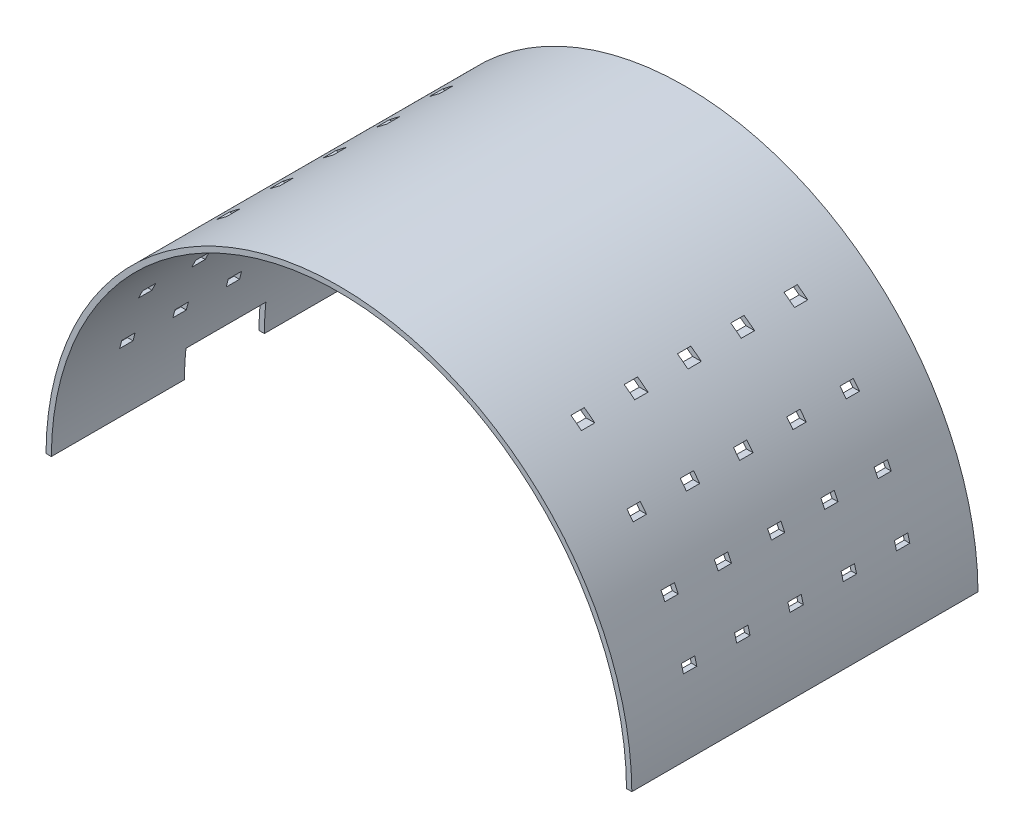
SolidWorks part; units mm, degrees
ref_plane "前视基准面" through (0, 0, 0) normal (0, 0, 1) x (1, 0, 0)
ref_plane "上视基准面" through (0, 0, 0) normal (0, 1, 0) x (1, 0, 0)
ref_plane "右视基准面" through (0, 0, 0) normal (1, 0, 0) x (0, 0, -1)
other "Configuration Table"
sketch "草图1" plane through (0, 0, 0) normal (0, 0, 1) x (1, 0, 0)
  line L0 (0.0023, 1) -> (4.0023, 1)
  line L1 (435.9977, 1) -> (439.9977, 1)
  arc A0 (439.9977, 1) -> (0.0023, 1) centre (220, 0) ccw
  arc A1 (4.0023, 1) -> (435.9977, 1) centre (220, 0) cw
  point P0 (0, 0)
  dimension "D1" = 220
  dimension "D2" = 216
  dimension "D3" = 4
extrude "凸台-拉伸1" add sketch "草图1" against normal mid plane 260
sketch "草图2" plane through (0, 0, 0) normal (1, 0, 0) x (0, 0, -1)
  line L0 (85, 52) -> (85, 58)
  line L1 (85, 58) -> (75, 58)
  line L2 (75, 58) -> (75, 52)
  line L3 (75, 52) -> (85, 52)
  line L4 (45, 52) -> (45, 58)
  line L5 (45, 58) -> (35, 58)
  line L6 (35, 58) -> (35, 52)
  line L7 (35, 52) -> (45, 52)
  line L8 (5, 52) -> (5, 58)
  line L9 (5, 58) -> (-5, 58)
  line L10 (-5, 58) -> (-5, 52)
  line L11 (-5, 52) -> (5, 52)
  line L12 (-35, 52) -> (-35, 58)
  line L13 (-35, 58) -> (-45, 58)
  line L14 (-45, 58) -> (-45, 52)
  line L15 (-45, 52) -> (-35, 52)
  line L16 (-75, 52) -> (-75, 58)
  line L17 (-75, 58) -> (-85, 58)
  line L18 (-85, 58) -> (-85, 52)
  line L19 (-85, 52) -> (-75, 52)
  line L20 (85, 92) -> (85, 98)
  line L21 (85, 98) -> (75, 98)
  line L22 (75, 98) -> (75, 92)
  line L23 (75, 92) -> (85, 92)
  line L24 (45, 92) -> (45, 98)
  line L25 (45, 98) -> (35, 98)
  line L26 (35, 98) -> (35, 92)
  line L27 (35, 92) -> (45, 92)
  line L28 (5, 92) -> (5, 98)
  line L29 (5, 98) -> (-5, 98)
  line L30 (-5, 98) -> (-5, 92)
  line L31 (-5, 92) -> (5, 92)
  line L32 (-35, 92) -> (-35, 98)
  line L33 (-35, 98) -> (-45, 98)
  line L34 (-45, 98) -> (-45, 92)
  line L35 (-45, 92) -> (-35, 92)
  line L36 (-75, 92) -> (-75, 98)
  line L37 (-75, 98) -> (-85, 98)
  line L38 (-85, 98) -> (-85, 92)
  line L39 (-85, 92) -> (-75, 92)
  line L40 (85, 132) -> (85, 138)
  line L41 (85, 138) -> (75, 138)
  line L42 (75, 138) -> (75, 132)
  line L43 (75, 132) -> (85, 132)
  line L44 (45, 132) -> (45, 138)
  line L45 (45, 138) -> (35, 138)
  line L46 (35, 138) -> (35, 132)
  line L47 (35, 132) -> (45, 132)
  line L48 (5, 132) -> (5, 138)
  line L49 (5, 138) -> (-5, 138)
  line L50 (-5, 138) -> (-5, 132)
  line L51 (-5, 132) -> (5, 132)
  line L52 (-35, 132) -> (-35, 138)
  line L53 (-35, 138) -> (-45, 138)
  line L54 (-45, 138) -> (-45, 132)
  line L55 (-45, 132) -> (-35, 132)
  line L56 (-75, 132) -> (-75, 138)
  line L57 (-75, 138) -> (-85, 138)
  line L58 (-85, 138) -> (-85, 132)
  line L59 (-85, 132) -> (-75, 132)
  line L60 (85, 172) -> (85, 178)
  line L61 (85, 178) -> (75, 178)
  line L62 (75, 178) -> (75, 172)
  line L63 (75, 172) -> (85, 172)
  line L64 (45, 172) -> (45, 178)
  line L65 (45, 178) -> (35, 178)
  line L66 (35, 178) -> (35, 172)
  line L67 (35, 172) -> (45, 172)
  line L68 (5, 172) -> (5, 178)
  line L69 (5, 178) -> (-5, 178)
  line L70 (-5, 178) -> (-5, 172)
  line L71 (-5, 172) -> (5, 172)
  line L72 (-35, 172) -> (-35, 178)
  line L73 (-35, 178) -> (-45, 178)
  line L74 (-45, 178) -> (-45, 172)
  line L75 (-45, 172) -> (-35, 172)
  line L76 (-75, 172) -> (-75, 178)
  line L77 (-75, 178) -> (-85, 178)
  line L78 (-85, 178) -> (-85, 172)
  line L79 (-85, 172) -> (-75, 172)
  point P0 (0, 0)
  dimension "D1" = 10
  dimension "D2" = 40
  dimension "D3" = 50
  dimension "D4" = 80
  dimension "D5" = 85
  dimension "D6" = 90
  dimension "D7" = 120
  dimension "D8" = 130
  dimension "D9" = 160
  dimension "D10" = 170
  dimension "D11" = 6
  dimension "D12" = 40
  dimension "D13" = 46
  dimension "D14" = 80
  dimension "D15" = 86
  dimension "D16" = 120
  dimension "D17" = 126
  dimension "D18" = 178
extrude "切除-拉伸1" cut sketch "草图2" against normal mid plane 1000
sketch "草图3" plane through (0, 0, 0) normal (0, 0, 1) x (1, 0, 0)
  line L0 (-10, -2) -> (30, -2)
  line L1 (30, -2) -> (30, 22)
  line L2 (30, 22) -> (-10, 22)
  line L3 (-10, 22) -> (-10, -2)
  point P0 (0, 0)
  dimension "D1" = 30
  dimension "D2" = 40
  dimension "D3" = 22
  dimension "D4" = 24
extrude "切除-拉伸2" cut sketch "草图3" against normal mid plane 60
